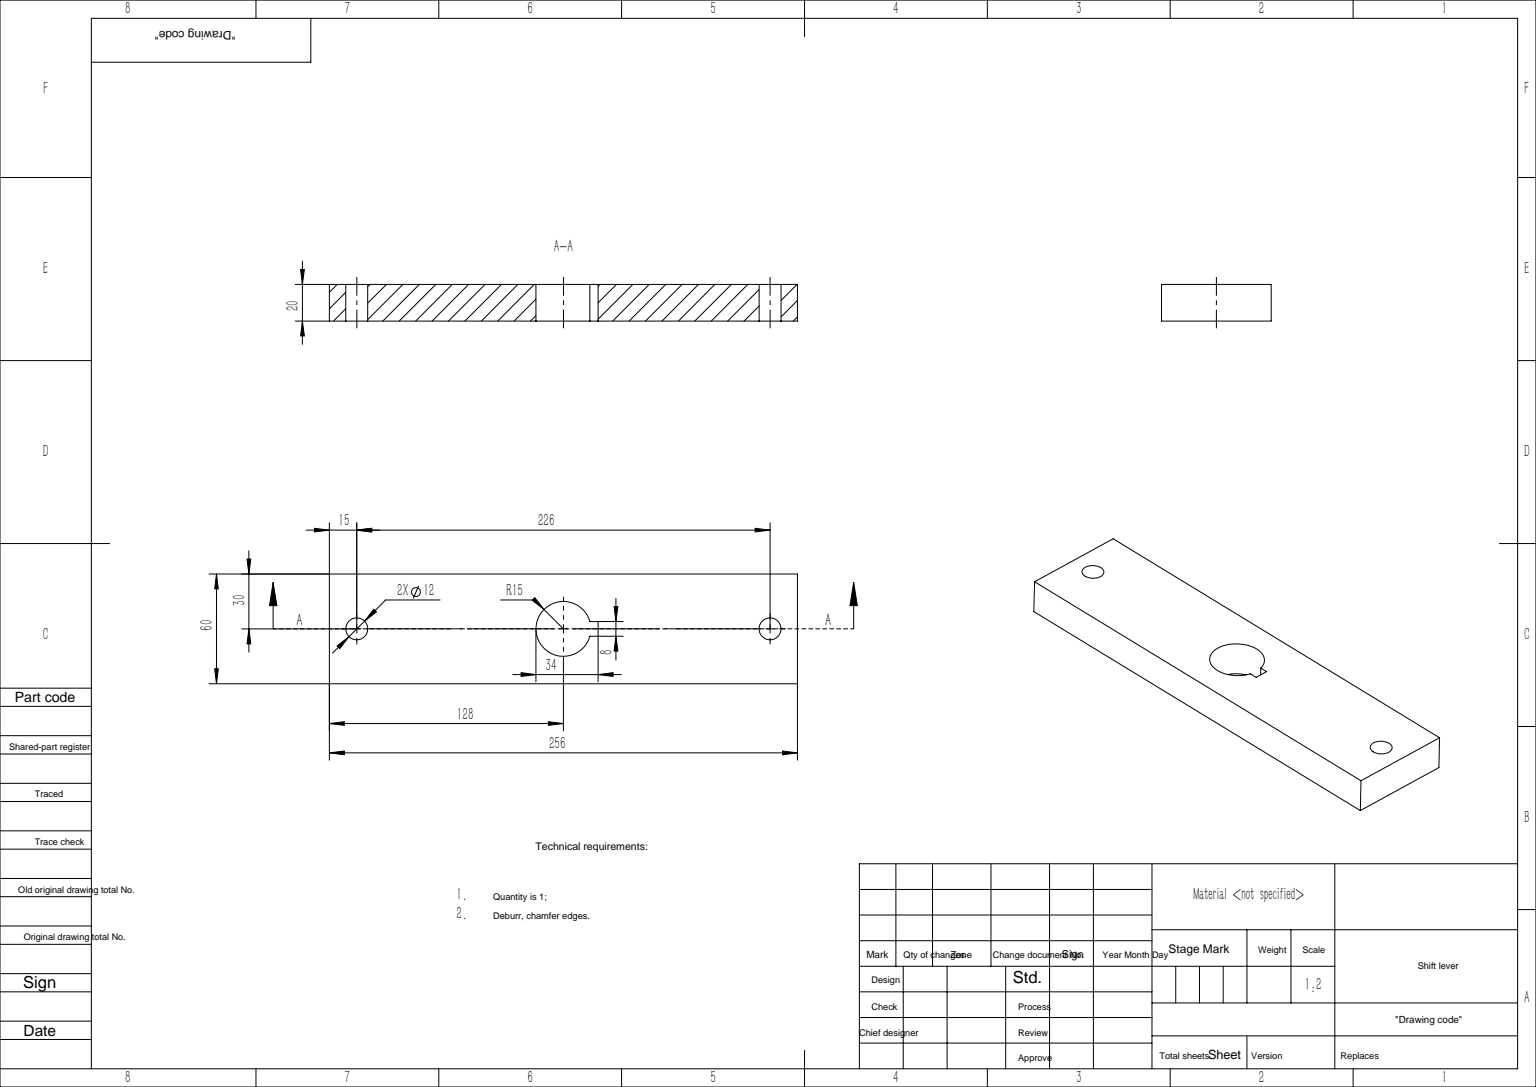
from build123d import *

# Parameters (mm, degrees)
SKETCH_1_W          = 60
SKETCH_1_H          = 256
EXTRUDE_1_DEPTH     = 20
SKETCH_2_R          = 6
CUT_EXTRUDE_1_DEPTH = 133.981201679
CUT_EXTRUDE_2_DEPTH = 133.981201679


with BuildPart() as part:
    # 草图1 → 凸台-拉伸1 (new body)
    with BuildSketch(Plane.XY):
        Rectangle(SKETCH_1_W, SKETCH_1_H)
    extrude(amount=EXTRUDE_1_DEPTH)

    # 草图2 → 切除-拉伸1 (cut, through all)
    with BuildSketch(Plane.XY.offset(20)):
        with Locations((0, 113)):
            Circle(SKETCH_2_R)
        with Locations((0, -113)):
            Circle(SKETCH_2_R)
    extrude(amount=-CUT_EXTRUDE_1_DEPTH, mode=Mode.SUBTRACT)

    # 草图3 → 切除-拉伸2 (cut, through all)
    with BuildSketch(Plane.XY.offset(20)):
        with BuildLine():
            Line((-4, 19), (4, 19))
            Line((4, 19), (4, 14.456832295))
            ThreePointArc((4, 14.456832295), (0, -15), (-4, 14.456832295))
            Line((-4, 14.456832295), (-4, 19))
        make_face()
    extrude(amount=-CUT_EXTRUDE_2_DEPTH, mode=Mode.SUBTRACT)


solid = part.part
